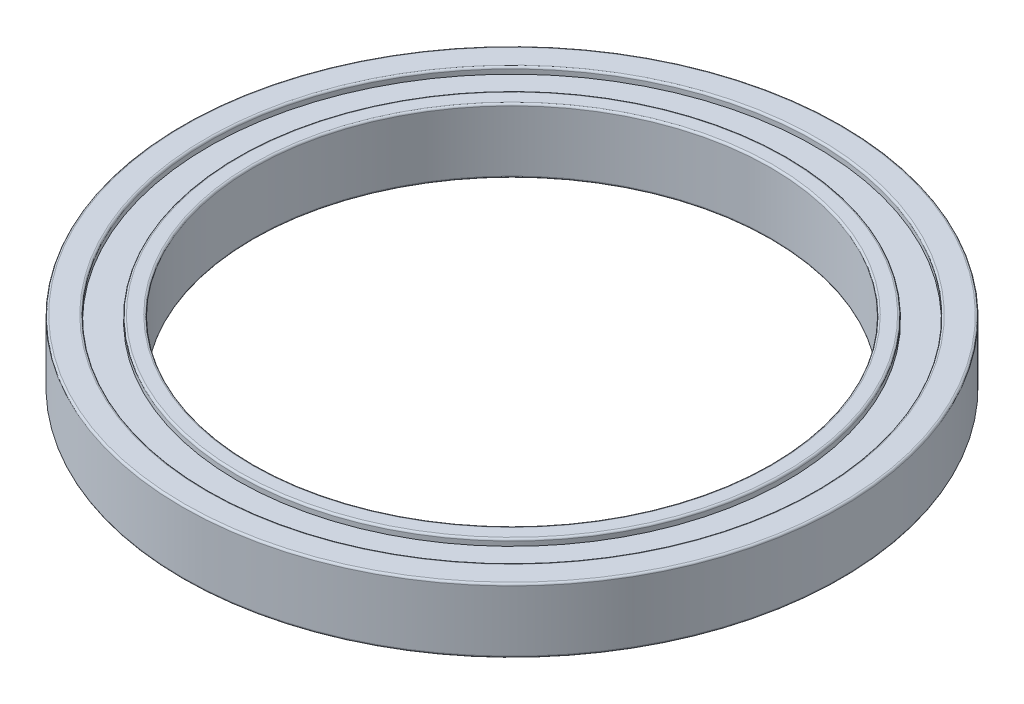
from build123d import *

# Parameters (mm, degrees)
SKETCH_1_R            = 25.5
SKETCH_1_R_2          = 20
EXTRUDE_1_DEPTH       = 2.5
SKETCH_2_R            = 23.5
SKETCH_2_R_2          = 21.25
CUT_EXTRUDE_433_DEPTH = 0.5
CUT_EXTRUDE_START     = -0.5
SKETCH_3_R            = 23.5
SKETCH_3_R_2          = 21.25
CUT_EXTRUDE_567_DEPTH = 0.5
SKETCH_4_R            = 0.75
CUT_EXTRUDE_START_2   = -22.35
SKETCH_5_R            = 0.5
CUT_EXTRUDE_1_DEPTH   = 14.79899722
FILLET_R0_15_R        = 0.15


with BuildPart() as part:
    # 草图1 → 凸台-拉伸1 (new, symmetric)
    with BuildSketch(Plane(origin=(0, 0, 0), x_dir=(1, 0, 0), z_dir=(0, 1, 0))):
        with Locations(Location((0, 0, 0), (0, 0, 270))):
            Circle(SKETCH_1_R)
        with Locations(Location((0, 0, 0), (0, 0, 270))):
            Circle(SKETCH_1_R_2, mode=Mode.SUBTRACT)
    extrude(amount=EXTRUDE_1_DEPTH, both=True)

    # 草图2 → Cut-Extrude 433 (cut)
    with BuildSketch(Plane(origin=(0, 2.5, 0), x_dir=(1, 0, 0), z_dir=(0, 1, 0))):
        with Locations(Location((0, 0, 0), (0, 0, 270))):
            Circle(SKETCH_2_R)
        with Locations(Location((0, 0, 0), (0, 0, 270))):
            Circle(SKETCH_2_R_2, mode=Mode.SUBTRACT)
    extrude(amount=-CUT_EXTRUDE_433_DEPTH, mode=Mode.SUBTRACT)

    # 草图3 → Cut-Extrude 567 (cut)
    with BuildSketch(Plane.XZ.offset(2.5).offset(CUT_EXTRUDE_START)):
        with Locations(Location((0, 0, 0), (0, 0, 90))):
            Circle(SKETCH_3_R)
        with Locations(Location((0, 0, 0), (0, 0, 90))):
            Circle(SKETCH_3_R_2, mode=Mode.SUBTRACT)
    extrude(amount=CUT_EXTRUDE_567_DEPTH, mode=Mode.SUBTRACT)

    # 草图4 → Cut-Revolve 663 (revolve, cut)
    with BuildSketch(Plane.XY, mode=Mode.PRIVATE) as cut_revolve_663_sk:
        with Locations((-22.35, 0)):
            Circle(SKETCH_4_R)
    revolve(cut_revolve_663_sk.sketch.rotate(Axis((0, 2.5, 0), (0, -1, 0)), 90), axis=Axis((0, 2.5, 0), (0, -1, 0)), mode=Mode.SUBTRACT)

    # 草图5 → 切除-拉伸1 (cut, through all)
    with BuildSketch(Plane.XY.offset(CUT_EXTRUDE_START_2)):
        with Locations(Location((0, 0, 0), (0, 0, 270))):
            Circle(SKETCH_5_R)
    extrude(amount=-CUT_EXTRUDE_1_DEPTH, mode=Mode.SUBTRACT)

    # R0.15 圆角
    fillet_r0_15_edges = [part.edges().sort_by_distance(p)[0] for p in [
        (0, 2.5, -23.5),
        (0, 2.5, -21.25),
        (0, -2.5, -23.5),
        (0, -2.5, -25.5),
        (0, -2.5, -21.25),
        (0, 2.5, -25.5),
        (0, -2.5, -20),
        (0, 2.5, -20),
    ]]
    fillet(fillet_r0_15_edges, radius=FILLET_R0_15_R)


solid = part.part
